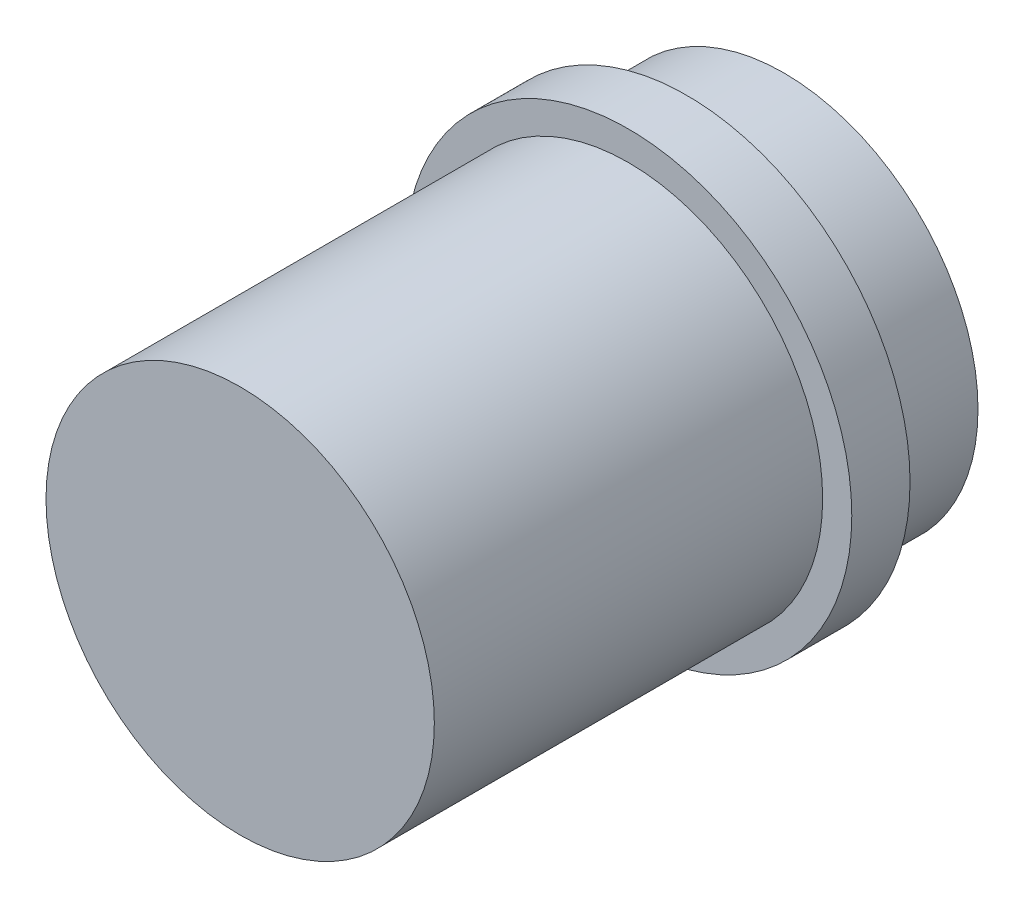
from build123d import *

# Parameters (mm, degrees)
SKETCH1_R           = 10
BOSS_EXTRUDE2_DEPTH = 5
SKETCH2_R           = 11.5
BOSS_EXTRUDE3_DEPTH = 3
SKETCH3_R           = 10
BOSS_EXTRUDE4_DEPTH = 20


with BuildPart() as part:
    # Sketch1 → Boss-Extrude2 (new body)
    with BuildSketch(Plane.XY):
        Circle(SKETCH1_R)
    extrude(amount=BOSS_EXTRUDE2_DEPTH)

    # Sketch2 → Boss-Extrude3 (add)
    with BuildSketch(Plane.XY.offset(5)):
        Circle(SKETCH2_R)
    extrude(amount=BOSS_EXTRUDE3_DEPTH)

    # Sketch3 → Boss-Extrude4 (add)
    with BuildSketch(Plane.XY.offset(8)):
        Circle(SKETCH3_R)
    extrude(amount=BOSS_EXTRUDE4_DEPTH)


solid = part.part
